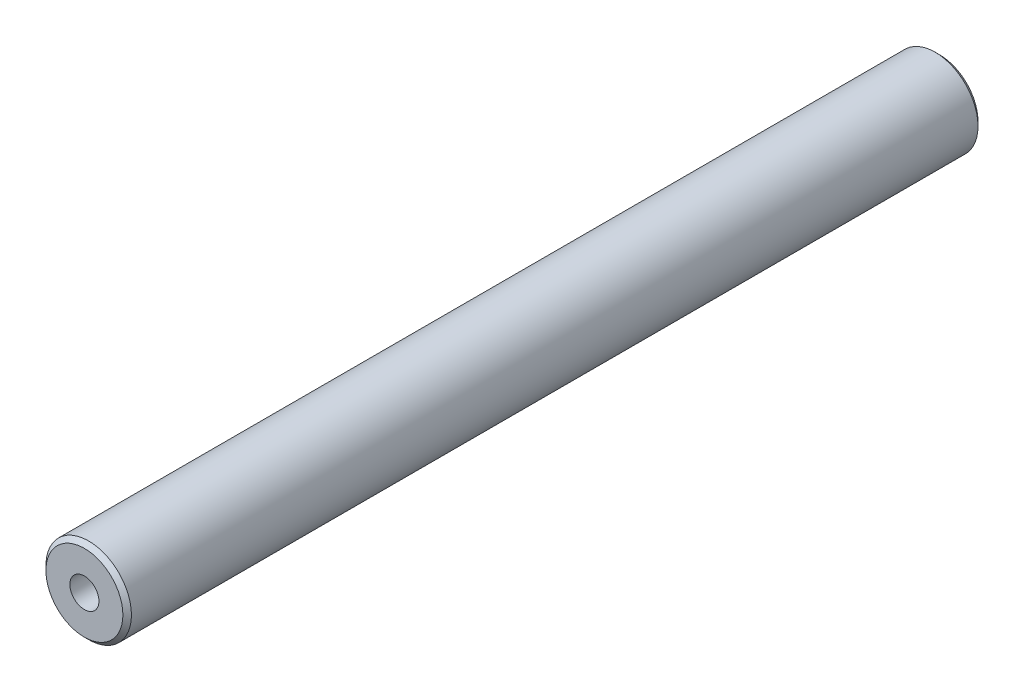
SolidWorks part; units mm, degrees
ref_plane "前视基准面" through (0, 0, 0) normal (0, 0, 1) x (1, 0, 0)
ref_plane "上视基准面" through (0, 0, 0) normal (0, 1, 0) x (1, 0, 0)
ref_plane "右视基准面" through (0, 0, 0) normal (1, 0, 0) x (0, 0, -1)
sketch "草图1" plane through (0, 0, 0) normal (0, 0, 1) x (1, 0, 0)
  circle A0 centre (0, 0) radius 10
  dimension "D1" = 20
extrude "凸台-拉伸1" add sketch "草图1" along normal blind 200
hole_wizard "M8 螺纹孔1" positions "草图2" profile "草图3" tap size "M8" standard "GB"
sketch "草图2" plane through (0, 0, 0) normal (0, 0, -1) x (-1, 0, 0)
  point P0 (0, 0)
sketch "草图3" plane through (0, 0, 0) normal (1, 0, 0) x (0, 1, 0)
  line L0 (0, 0) -> (0, 21.7929)
  line L1 (0, 21.7929) -> (3.4, 19.75)
  line L2 (3.4, 19.75) -> (3.4, 0)
  line L5 (3.4, 0) -> (0, 0)
  line L10 (0, 21.7929) -> (-3.4, 19.75) construction
  line L11 (0, -6.35) -> (0, 107.95) construction
  dimension "螺纹孔钻头直径" = 6.8
  dimension "螺纹孔钻头深度" = 19.75
  dimension "导头角度" = 118
cosmetic thread "孔螺蚊线1"
hole_wizard "M8 螺纹孔2" positions "草图4" profile "草图5" tap size "M8" standard "GB"
sketch "草图4" plane through (0, 0, 200) normal (0, 0, 1) x (1, 0, 0)
  point P0 (0, 0)
sketch "草图5" plane through (0, 0, 200) normal (1, 0, 0) x (0, -1, 0)
  line L0 (0, 0) -> (0, 21.7929)
  line L1 (0, 21.7929) -> (3.4, 19.75)
  line L2 (3.4, 19.75) -> (3.4, 0)
  line L5 (3.4, 0) -> (0, 0)
  line L10 (0, 21.7929) -> (-3.4, 19.75) construction
  line L11 (0, -6.35) -> (0, 107.95) construction
  dimension "螺纹孔钻头直径" = 6.8
  dimension "螺纹孔钻头深度" = 19.75
  dimension "导头角度" = 118
cosmetic thread "孔螺蚊线2"
chamfer "倒角1" distance 1 angle 45 2 edges at (10, 0, 0) (10, 0, 200)
